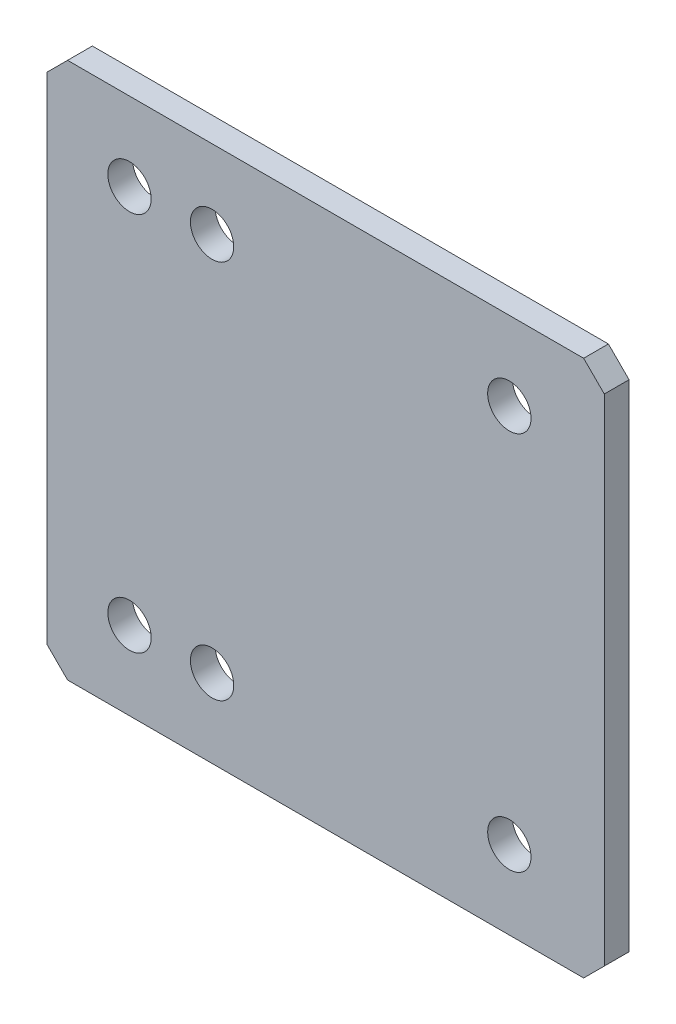
SolidWorks part; units mm, degrees
material "1023 碳钢板 (SS)"
ref_plane "Front Plane" through (0, 0, 0) normal (0, 0, 1) x (1, 0, 0)
ref_plane "Top Plane" through (0, 0, 0) normal (0, 1, 0) x (1, 0, 0)
ref_plane "Right Plane" through (0, 0, 0) normal (1, 0, 0) x (0, 0, -1)
sketch "Sketch1" plane through (0, 0, 0) normal (0, 0, 1) x (1, 0, 0)
  line L0 (-67.5, 60) -> (-62.5, 65)
  line L1 (62.5, -65) -> (-62.5, -65)
  line L2 (67.5, -60) -> (67.5, 60)
  line L3 (62.5, 65) -> (-62.5, 65)
  line L4 (-67.5, -60) -> (-67.5, 60)
  line L5 (67.5, -65) -> (-67.5, 65) construction
  line L6 (67.5, 65) -> (-67.5, -65) construction
  line L7 (67.5, 60) -> (62.5, 65)
  line L8 (62.5, -65) -> (67.5, -60)
  line L9 (-62.5, -65) -> (-67.5, -60)
  line L10 (-67.5, 0) -> (67.5, 0) construction
  circle A0 centre (-47.5, 46) radius 5.25
  circle A1 centre (-27.5, 46) radius 5.25
  circle A2 centre (44.5, 46) radius 5.25
  circle A3 centre (44.5, -46) radius 5.25
  circle A4 centre (-27.5, -46) radius 5.25
  circle A5 centre (-47.5, -46) radius 5.25
  point P0 (0, 0)
  dimension "D3" = 10.5
  dimension "D4" = 19
  dimension "D5" = 20
  dimension "D6" = 20
  dimension "D7" = 72
  dimension "D1" = 135
  dimension "D2" = 130
extrude "Boss-Extrude1" add sketch "Sketch1" along normal mid plane 6
